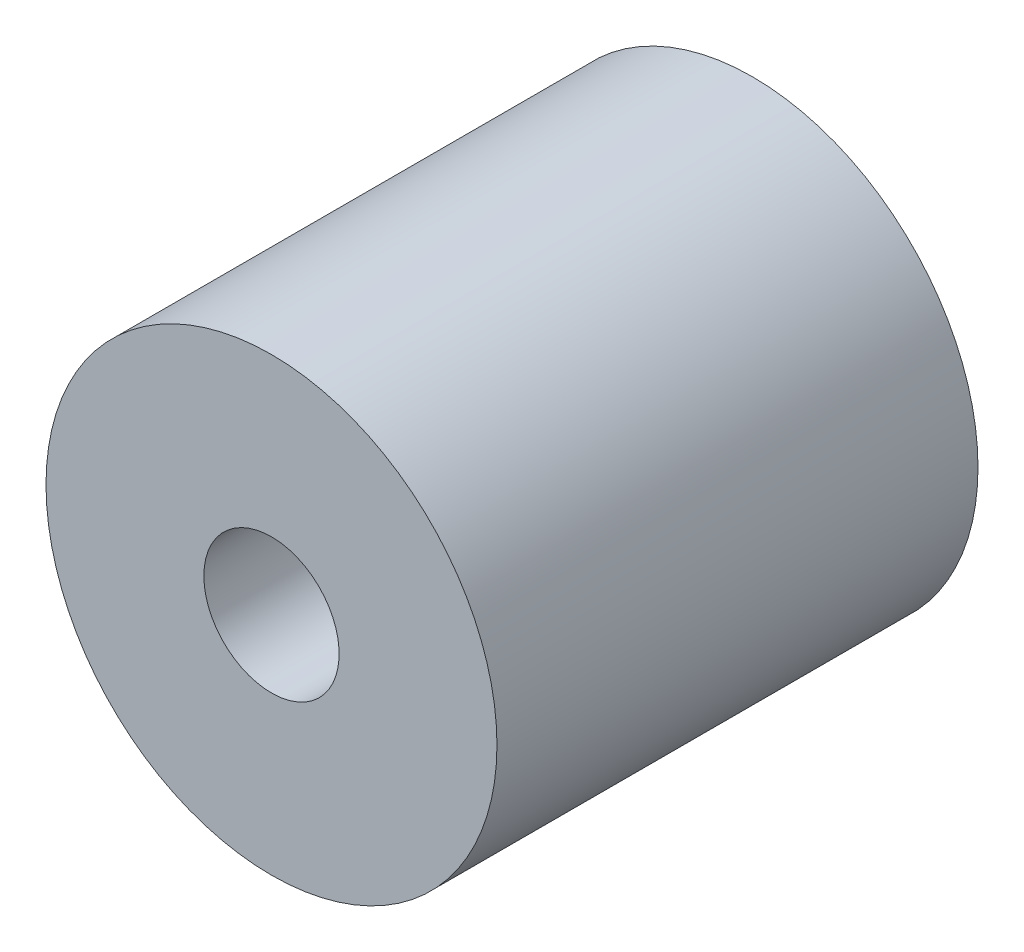
from build123d import *

# Parameters (mm, degrees)
SKETCH_1_R                   = 7.5
EXTRUDE_1_DEPTH              = 16
HOLE_WIZARD_M4_1_D           = 4.5
HOLE_WIZARD_M4_1_CBORE_D     = 9
HOLE_WIZARD_M4_1_CBORE_DEPTH = 12
CHAMFER_1_SIZE               = 1


with BuildPart() as part:
    # 草图1 → 凸台-拉伸1 (new body)
    with BuildSketch(Plane.XY):
        Circle(SKETCH_1_R)
    extrude(amount=EXTRUDE_1_DEPTH)

    # M4 六角凹头螺钉的柱形沉头孔1 (through all)
    with Locations(Plane(origin=(0, 0, 0), x_dir=(-1, 0, 0), z_dir=(0, 0, -1))):
        with Locations((0, 0)):
            CounterBoreHole(HOLE_WIZARD_M4_1_D / 2, HOLE_WIZARD_M4_1_CBORE_D / 2, HOLE_WIZARD_M4_1_CBORE_DEPTH)

    # 倒角1
    chamfer_1_edges = [part.edges().sort_by_distance(p)[0] for p in [
        (4.5, 0, 0),
    ]]
    chamfer(chamfer_1_edges, length=CHAMFER_1_SIZE)


solid = part.part
